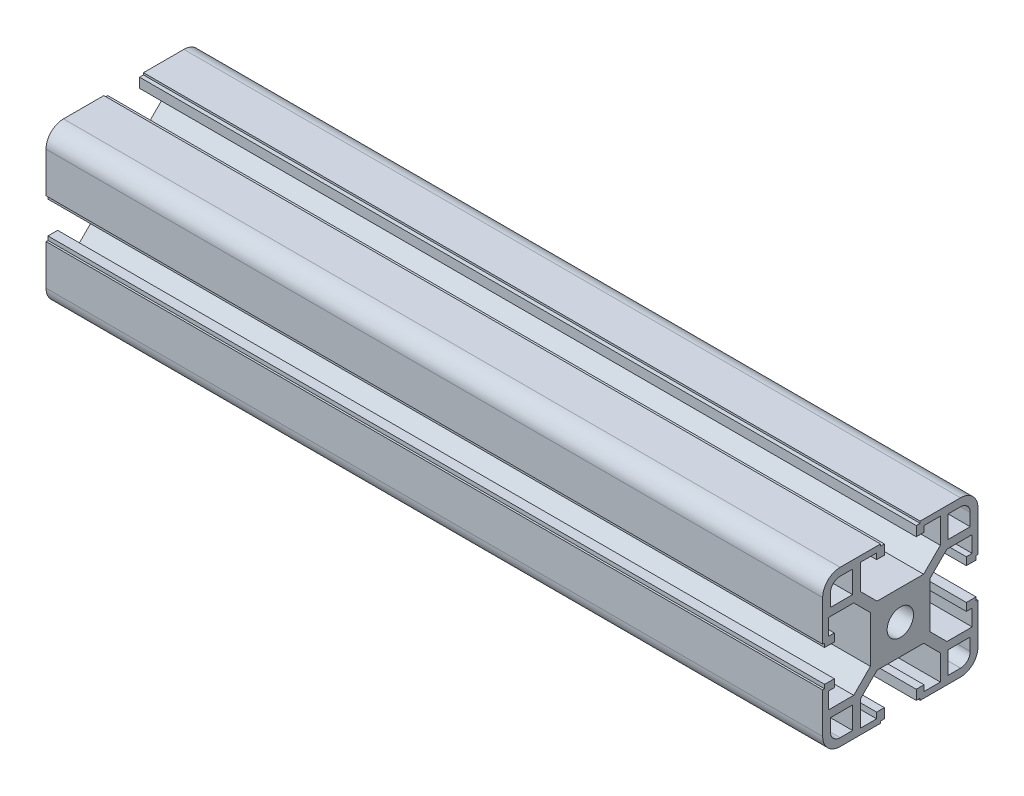
from build123d import *

# Parameters (mm, degrees)
SKETCH1_R                                 = 3.4
ALUMINIUM_PROFILE_40_X_40B_X_R4_5_1_DEPTH = 200


with BuildPart() as part:
    # Sketch1 → Aluminium profile 40 X 40B X R4.5(1) (new body)
    with BuildSketch(Plane.YZ.offset(-984.974958264)):
        with BuildLine():
            Line((-5.1, 20), (-5.1, 19.5))
            Line((-5.1, 19.5), (-4.1, 19.5))
            Line((-4.1, 19.5), (-4.1, 17))
            Line((-4.1, 17), (-6.1, 17))
            Line((-6.1, 17), (-6.1, 18.5))
            Line((-6.1, 18.5), (-10.3, 18.5))
            Line((-10.3, 18.5), (-10.3, 12))
            Line((-10.3, 12), (-6, 7.7))
            Line((-6, 7.7), (6, 7.7))
            Line((6, 7.7), (10.3, 12))
            Line((10.3, 12), (10.3, 18.5))
            Line((10.3, 18.5), (6.1, 18.5))
            Line((6.1, 18.5), (6.1, 17))
            Line((6.1, 17), (4.1, 17))
            Line((4.1, 17), (4.1, 19.5))
            Line((4.1, 19.5), (5.1, 19.5))
            Line((5.1, 19.5), (5.1, 20))
            Line((5.1, 20), (15.5, 20))
            ThreePointArc((15.5, 20), (18.681980515, 18.681980515), (20, 15.5))
            Line((20, 15.5), (20, 5.1))
            Line((20, 5.1), (19.5, 5.1))
            Line((19.5, 5.1), (19.5, 4.1))
            Line((19.5, 4.1), (17, 4.1))
            Line((17, 4.1), (17, 6.1))
            Line((17, 6.1), (18.5, 6.1))
            Line((18.5, 6.1), (18.5, 10.3))
            Line((18.5, 10.3), (12, 10.3))
            Line((12, 10.3), (7.7, 6))
            Line((7.7, 6), (7.7, -6))
            Line((7.7, -6), (12, -10.3))
            Line((12, -10.3), (18.5, -10.3))
            Line((18.5, -10.3), (18.5, -6.1))
            Line((18.5, -6.1), (17, -6.1))
            Line((17, -6.1), (17, -4.1))
            Line((17, -4.1), (19.5, -4.1))
            Line((19.5, -4.1), (19.5, -5.1))
            Line((19.5, -5.1), (20, -5.1))
            Line((20, -5.1), (20, -15.5))
            ThreePointArc((20, -15.5), (18.681980515, -18.681980515), (15.5, -20))
            Line((15.5, -20), (5.1, -20))
            Line((5.1, -20), (5.1, -19.5))
            Line((5.1, -19.5), (4.1, -19.5))
            Line((4.1, -19.5), (4.1, -17))
            Line((4.1, -17), (6.1, -17))
            Line((6.1, -17), (6.1, -18.5))
            Line((6.1, -18.5), (10.3, -18.5))
            Line((10.3, -18.5), (10.3, -12))
            Line((10.3, -12), (6, -7.7))
            Line((6, -7.7), (-6, -7.7))
            Line((-6, -7.7), (-10.3, -12))
            Line((-10.3, -12), (-10.3, -18.5))
            Line((-10.3, -18.5), (-6.1, -18.5))
            Line((-6.1, -18.5), (-6.1, -17))
            Line((-6.1, -17), (-4.1, -17))
            Line((-4.1, -17), (-4.1, -19.5))
            Line((-4.1, -19.5), (-5.1, -19.5))
            Line((-5.1, -19.5), (-5.1, -20))
            Line((-5.1, -20), (-15.5, -20))
            ThreePointArc((-15.5, -20), (-18.681980515, -18.681980515), (-20, -15.5))
            Line((-20, -15.5), (-20, -5.1))
            Line((-20, -5.1), (-19.5, -5.1))
            Line((-19.5, -5.1), (-19.5, -4.1))
            Line((-19.5, -4.1), (-17, -4.1))
            Line((-17, -4.1), (-17, -6.1))
            Line((-17, -6.1), (-18.5, -6.1))
            Line((-18.5, -6.1), (-18.5, -10.3))
            Line((-18.5, -10.3), (-12, -10.3))
            Line((-12, -10.3), (-7.7, -6))
            Line((-7.7, -6), (-7.7, 6))
            Line((-7.7, 6), (-12, 10.3))
            Line((-12, 10.3), (-18.5, 10.3))
            Line((-18.5, 10.3), (-18.5, 6.1))
            Line((-18.5, 6.1), (-17, 6.1))
            Line((-17, 6.1), (-17, 4.1))
            Line((-17, 4.1), (-19.5, 4.1))
            Line((-19.5, 4.1), (-19.5, 5.1))
            Line((-19.5, 5.1), (-20, 5.1))
            Line((-20, 5.1), (-20, 15.5))
            ThreePointArc((-20, 15.5), (-18.681980515, 18.681980515), (-15.5, 20))
            Line((-15.5, 20), (-5.1, 20))
        make_face()
        Circle(SKETCH1_R, mode=Mode.SUBTRACT)
        with BuildLine():
            Line((12.3, 18), (15.5, 18))
            ThreePointArc((15.5, 18), (17.267766953, 17.267766953), (18, 15.5))
            Line((18, 15.5), (18, 12.3))
            Line((18, 12.3), (12.3, 12.3))
            Line((12.3, 12.3), (12.3, 18))
        make_face(mode=Mode.SUBTRACT)
        with BuildLine():
            Line((-15.5, 18), (-12.3, 18))
            Line((-12.3, 18), (-12.3, 12.3))
            Line((-12.3, 12.3), (-18, 12.3))
            Line((-18, 12.3), (-18, 15.5))
            ThreePointArc((-18, 15.5), (-17.267766953, 17.267766953), (-15.5, 18))
        make_face(mode=Mode.SUBTRACT)
        with BuildLine():
            Line((-18, -12.3), (-12.3, -12.3))
            Line((-12.3, -12.3), (-12.3, -18))
            Line((-12.3, -18), (-15.5, -18))
            ThreePointArc((-15.5, -18), (-17.267766953, -17.267766953), (-18, -15.5))
            Line((-18, -15.5), (-18, -12.3))
        make_face(mode=Mode.SUBTRACT)
        with BuildLine():
            Line((12.3, -12.3), (18, -12.3))
            Line((18, -12.3), (18, -15.5))
            ThreePointArc((18, -15.5), (17.267766953, -17.267766953), (15.5, -18))
            Line((15.5, -18), (12.3, -18))
            Line((12.3, -18), (12.3, -12.3))
        make_face(mode=Mode.SUBTRACT)
    extrude(amount=ALUMINIUM_PROFILE_40_X_40B_X_R4_5_1_DEPTH)


solid = part.part
